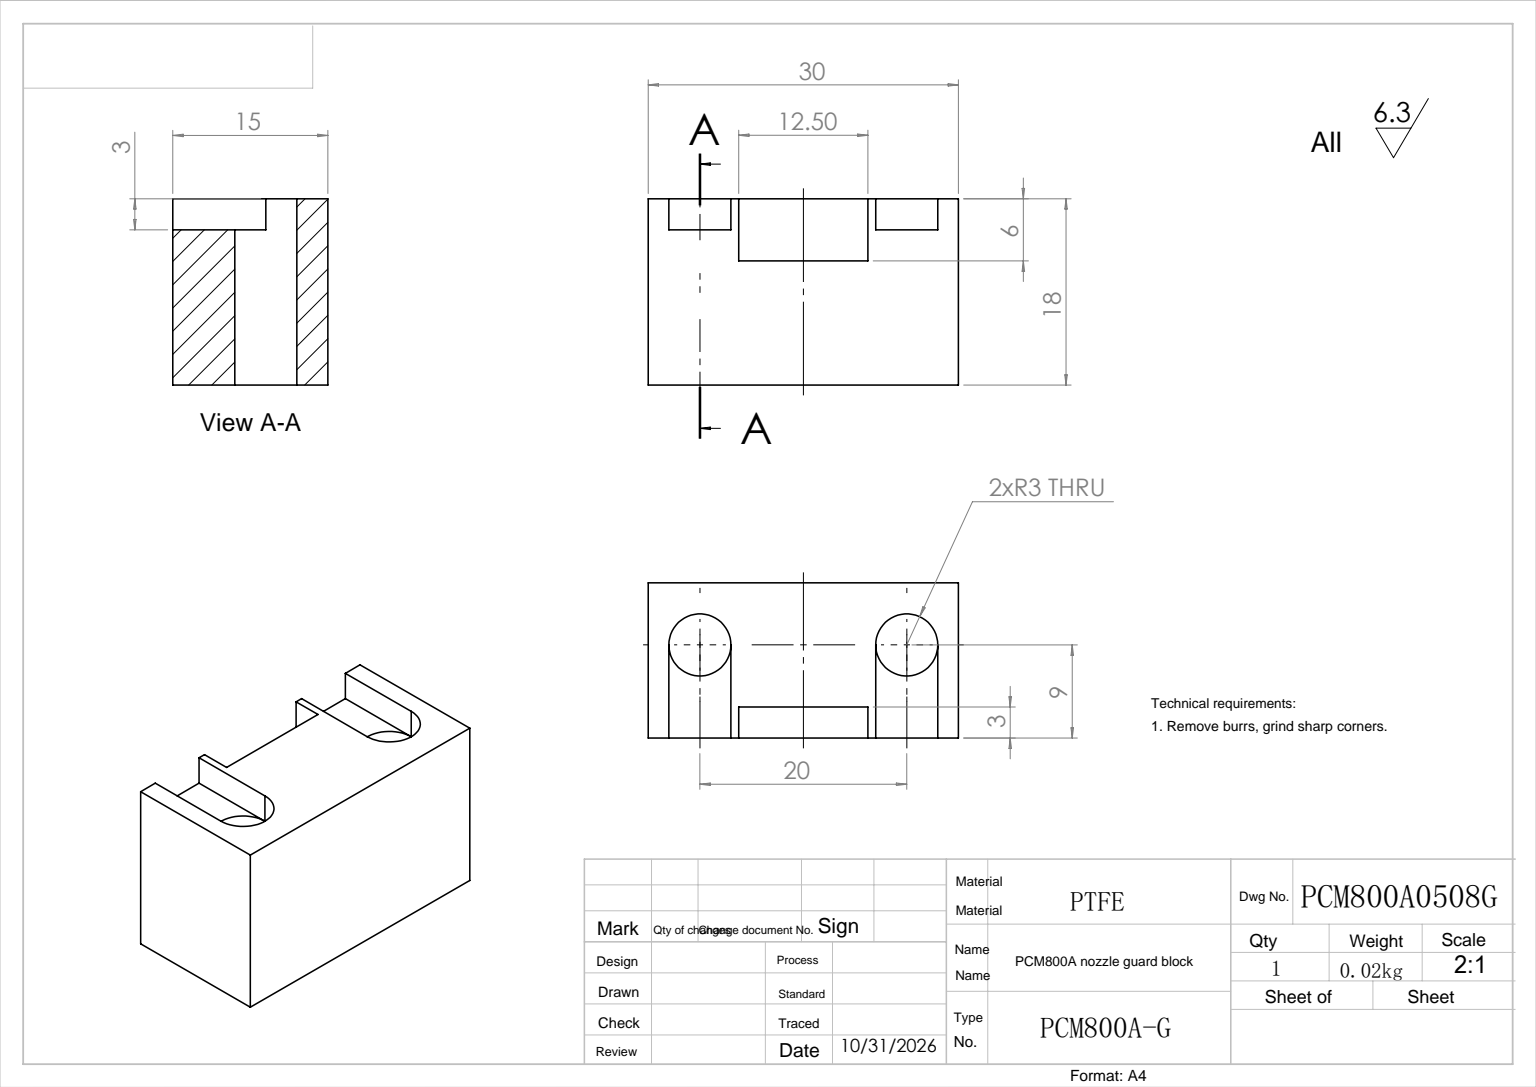
from build123d import *

# Parameters (mm, degrees)
SKETCH_1_W             = 15
SKETCH_1_H             = 18
EXTRUDE_1_DEPTH        = 30
SKETCH_2_R             = 3
CUT_EXTRUDE_1_DEPTH    = 39.065732621
CUT_EXTRUDE_3_DEPTH    = 3
PATTERN_LINEAR_1_COUNT = 2
PATTERN_LINEAR_1_PITCH = 20
SKETCH_5_W             = 6
SKETCH_5_H             = 12.5
CUT_EXTRUDE_4_DEPTH    = 3


with BuildPart() as part:
    # 草图1 → 拉伸1 (new body)
    with BuildSketch(Plane.XY):
        with Locations((7.5, 9)):
            Rectangle(SKETCH_1_W, SKETCH_1_H)
    extrude(amount=EXTRUDE_1_DEPTH)

    # 草图2 → 切除-拉伸1 (cut, through all)
    with BuildSketch(Plane(origin=(0, 18, 0), x_dir=(-1, 0, 0), z_dir=(0, 1, 0))):
        with Locations(Location((-6, 5, 0), (0, 0, 90))):
            Circle(SKETCH_2_R)
    cut_extrude_1 = extrude(amount=-CUT_EXTRUDE_1_DEPTH, mode=Mode.SUBTRACT)

    # 草图4 → 切除-拉伸3 (cut)
    with BuildSketch(Plane(origin=(0, 18, 0), x_dir=(-1, 0, 0), z_dir=(0, 1, 0))):
        with BuildLine():
            Line((-15, 2), (-6, 2))
            ThreePointArc((-6, 2), (-3, 5), (-6, 8))
            Line((-6, 8), (-15, 8))
            Line((-15, 8), (-15, 2))
        make_face()
    cut_extrude_3 = extrude(amount=-CUT_EXTRUDE_3_DEPTH, mode=Mode.SUBTRACT)

    # 阵列(线性)1: 切除-拉伸1, 切除-拉伸3 ×2
    with Locations(*[(0, 0, i * PATTERN_LINEAR_1_PITCH) for i in range(1, PATTERN_LINEAR_1_COUNT)]):
        add(cut_extrude_1, mode=Mode.SUBTRACT)
        add(cut_extrude_3, mode=Mode.SUBTRACT)

    # 草图5 → 切除-拉伸4 (cut)
    with BuildSketch(Plane(origin=(15, 3, 0), x_dir=(0, 1, 0), z_dir=(-1, 0, 0))):
        with Locations((12, -15)):
            Rectangle(SKETCH_5_W, SKETCH_5_H)
    extrude(amount=CUT_EXTRUDE_4_DEPTH, mode=Mode.SUBTRACT)


solid = part.part
